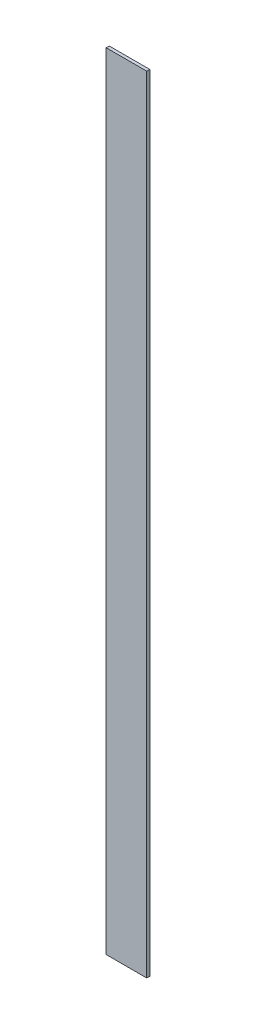
SolidWorks part; units mm, degrees
material "普通碳钢"
ref_plane "Front Plane" through (0, 0, 0) normal (0, 0, 1) x (1, 0, 0)
ref_plane "Top Plane" through (0, 0, 0) normal (0, 1, 0) x (1, 0, 0)
ref_plane "Right Plane" through (0, 0, 0) normal (1, 0, 0) x (0, 0, -1)
sketch "Sketch1" plane through (0, 0, 0) normal (0, 0, 1) x (1, 0, 0)
  line L1 (-200, 3878) -> (200, 3878)
  line L2 (-200, 3878) -> (-200, -3878)
  line L3 (-200, -3878) -> (200, -3878)
  line L4 (200, 3878) -> (200, -3878)
  dimension "D1" = 7756
  dimension "D2" = 400
  dimension "D3" = 3878
  dimension "D4" = 200
extrude "Boss-Extrude1" add sketch "Sketch1" along normal mid plane 30
